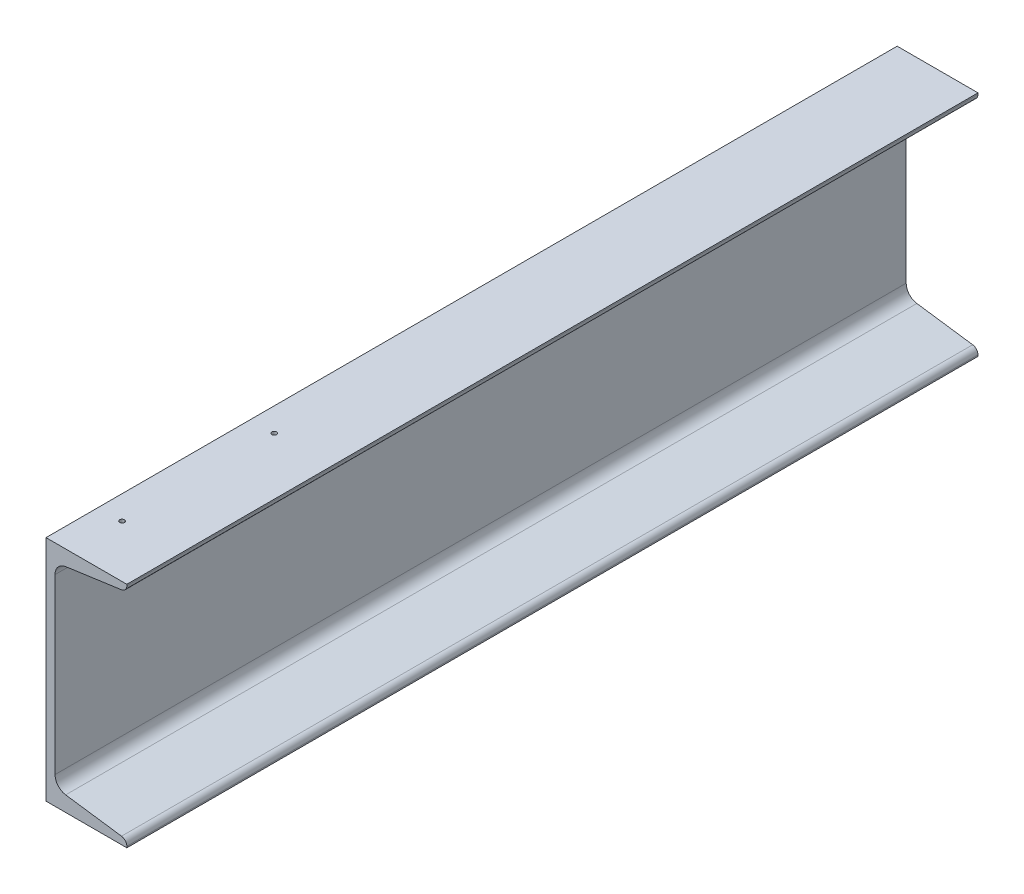
SolidWorks part; units mm, degrees
material "1023 碳钢板 (SS)"
ref_plane "前视基准面" through (0, 0, 0) normal (0, 0, 1) x (1, 0, 0)
ref_plane "上视基准面" through (0, 0, 0) normal (0, 1, 0) x (1, 0, 0)
ref_plane "右视基准面" through (0, 0, 0) normal (1, 0, 0) x (0, 0, -1)
sketch "草图1" plane through (0, 0, 0) normal (0, 0, 1) x (1, 0, 0)
  line L0 (0, 0) -> (-85, 0)
  line L1 (-85, 0) -> (-85, -240)
  line L2 (-85, -240) -> (0, -240)
  line L3 (0, -240) -> (0, -238.6233)
  line L4 (-5.5954, -232.1866) -> (-64.3093, -223.9349)
  line L5 (-75.5, -211.0614) -> (-75.5, -28.9386)
  line L6 (-64.3093, -16.0651) -> (-5.5954, -7.8134)
  line L7 (0, -1.3767) -> (0, 0)
  line L8 (-42.5, -227) -> (-42.5, -240) construction
  arc A0 (-64.3093, -223.9349) -> (-75.5, -211.0614) centre (-62.5, -211.0614) cw
  arc A1 (-75.5, -28.9386) -> (-64.3093, -16.0651) centre (-62.5, -28.9386) cw
  arc A2 (0, -238.6233) -> (-5.5954, -232.1866) centre (-6.5, -238.6233) ccw
  arc A3 (-5.5954, -7.8134) -> (0, -1.3767) centre (-6.5, -1.3767) ccw
  dimension "D7" = 13
  dimension "D8" = 6.5
  dimension "D1" = 240
  dimension "D2" = 85
  dimension "D3" = 42.5
  dimension "D4" = 13
  dimension "D5" = 9.5
  dimension "D6" = 8
extrude "凸台-拉伸1" add sketch "草图1" along normal blind 895 contours A3 L6 A1 L5 A0 L4 A2 L3 L2 L1 L0 L7
sketch "草图2" plane through (-85, 0, 0) normal (-1, 0, 0) x (0, 0, 1)
  line L0 (895, 0) -> (0, 0) construction
  line L2 (0, -211.0614) -> (0, -28.9386) construction
  circle A0 centre (2840, -126) radius 10
  circle A1 centre (2840, -196) radius 10
  circle A2 centre (2640, -126) radius 10
  circle A3 centre (2640, -196) radius 10
  circle A4 centre (2440, -126) radius 10
  circle A5 centre (2440, -196) radius 10
  circle A6 centre (2240, -126) radius 10
  circle A7 centre (2240, -196) radius 10
  circle A8 centre (2040, -126) radius 10
  circle A9 centre (2040, -196) radius 10
  circle A10 centre (1840, -126) radius 10
  circle A11 centre (1840, -196) radius 10
  circle A12 centre (1640, -126) radius 10
  circle A13 centre (1640, -196) radius 10
  circle A14 centre (1440, -126) radius 10
  circle A15 centre (1440, -196) radius 10
  circle A16 centre (1240, -126) radius 10
  circle A17 centre (1240, -196) radius 10
  circle A18 centre (1040, -126) radius 10
  circle A19 centre (1040, -196) radius 10
  circle A20 centre (840, -126) radius 10
  circle A21 centre (840, -196) radius 10
  circle A22 centre (640, -126) radius 10
  circle A23 centre (640, -196) radius 10
  circle A24 centre (440, -126) radius 10
  circle A25 centre (440, -196) radius 10
  circle A26 centre (240, -126) radius 10
  circle A27 centre (240, -196) radius 10
  dimension "D3" = 240
  dimension "D4" = 20
  dimension "D1" = 70
  dimension "D2" = 126
  dimension "D5" = 14
sketch "草图6" plane through (-85, 0, 0) normal (-1, 0, 0) x (0, 0, 1)
  line L0 (895, 0) -> (0, 0) construction
  line L1 (0, 0) -> (0, -240) construction
  circle A0 centre (630, -50) radius 25.9537
  circle A1 centre (710, -50) radius 27.9359
  dimension "D3" = 630
  dimension "D1" = 80
  dimension "D2" = 50
hole_wizard "M8 螺纹孔1" positions "草图7" profile "草图8" tap size "M8" standard "ISO"
sketch "草图7" plane through (-85, 0, 0) normal (-1, 0, 0) x (0, 0, 1)
  point P0 (630, -50)
  point P3 (710, -50)
sketch "草图8" plane through (-85, -50, 630) normal (0, 1, 0) x (0, 0, 1)
  line L0 (0, 0) -> (0, 21.7929)
  line L1 (0, 21.7929) -> (3.4, 19.75)
  line L2 (3.4, 19.75) -> (3.4, 0)
  line L5 (3.4, 0) -> (0, 0)
  line L10 (0, 21.7929) -> (-3.4, 19.75) construction
  line L11 (0, -6.35) -> (0, 107.95) construction
  dimension "螺纹孔钻头直径" = 6.8
  dimension "螺纹孔钻头深度" = 19.75
  dimension "导头角度" = 118
cosmetic thread "孔螺蚊线1" parameters "D1"=16, "D2"=8
cosmetic thread "孔螺蚊线2" parameters "D1"=16, "D2"=8
sketch "草图9" plane through (0, 0, 0) normal (0, 1, 0) x (1, 0, 0)
  line L0 (0, 0) -> (-85, 0) construction
  line L1 (-85, -895) -> (-85, 0) construction
  circle A0 centre (-60, -680) radius 6
  circle A1 centre (-60, -840) radius 6
  point P8 (0, 0)
  dimension "D2" = 680
  dimension "D3" = 25
  dimension "D4" = 12
  dimension "D1" = 160
hole_wizard "M6 螺纹孔1" positions "草图10" profile "草图11" tap size "M6" standard "ISO"
sketch "草图10" plane through (0, 0, 0) normal (0, 1, 0) x (1, 0, 0)
  point P0 (-60, -840)
  point P3 (-60, -680)
sketch "草图11" plane through (-60, 0, 840) normal (1, 0, 0) x (0, 0, 1)
  line L0 (0, 0) -> (0, 16.5022)
  line L1 (0, 16.5022) -> (2.5, 15)
  line L2 (2.5, 15) -> (2.5, 0)
  line L5 (2.5, 0) -> (0, 0)
  line L10 (0, 16.5022) -> (-2.5, 15) construction
  line L11 (0, -6.35) -> (0, 107.95) construction
  dimension "螺纹孔钻头直径" = 5
  dimension "螺纹孔钻头深度" = 15
  dimension "导头角度" = 118
cosmetic thread "孔螺蚊线3" parameters "D1"=12, "D2"=6
cosmetic thread "孔螺蚊线4" parameters "D1"=12, "D2"=6
